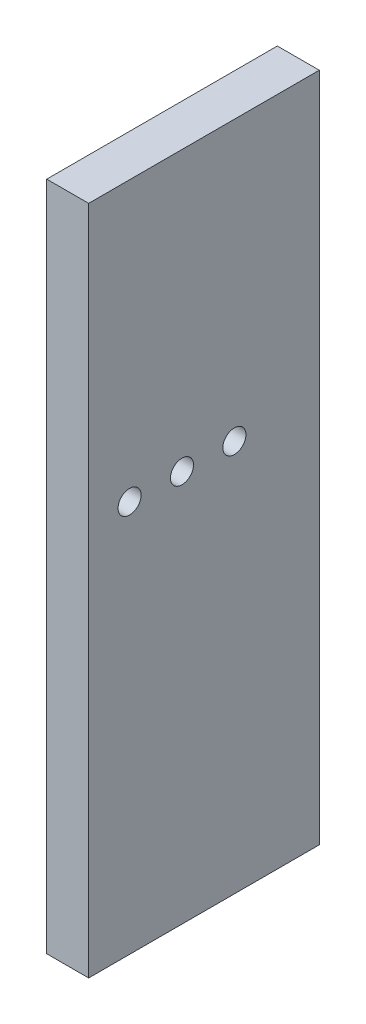
from build123d import *

# Parameters (mm, degrees)
SKETCH1_W                                = 20
SKETCH1_H                                = 320
BOSS_EXTRUDE1_DEPTH                      = 110
CBORE_FOR_M10_HEX_HEAD_BOLT1_D           = 11
CBORE_FOR_M10_HEX_HEAD_BOLT1_DEPTH       = 22.25
CBORE_FOR_M10_HEX_HEAD_BOLT1_CBORE_D     = 15
CBORE_FOR_M10_HEX_HEAD_BOLT1_CBORE_DEPTH = 10
CBORE_FOR_M10_HEX_HEAD_BOLT1_TIP         = 3.304733405


with BuildPart() as part:
    # Sketch1 → Boss-Extrude1 (new body)
    with BuildSketch(Plane.XY):
        with Locations((-110, 300)):
            Rectangle(SKETCH1_W, SKETCH1_H)
    extrude(amount=BOSS_EXTRUDE1_DEPTH)

    # CBORE for M10 Hex Head Bolt1
    with Locations(Plane.ZY.offset(120)):
        with Locations((40.49, 327), (65.49, 327), (90.49, 327)):
            CounterBoreHole(CBORE_FOR_M10_HEX_HEAD_BOLT1_D / 2, CBORE_FOR_M10_HEX_HEAD_BOLT1_CBORE_D / 2, CBORE_FOR_M10_HEX_HEAD_BOLT1_CBORE_DEPTH, depth=CBORE_FOR_M10_HEX_HEAD_BOLT1_DEPTH)
            with Locations((0, 0, -(CBORE_FOR_M10_HEX_HEAD_BOLT1_DEPTH + CBORE_FOR_M10_HEX_HEAD_BOLT1_TIP / 2))):  # 118° drill point
                Cone(0, CBORE_FOR_M10_HEX_HEAD_BOLT1_D / 2, CBORE_FOR_M10_HEX_HEAD_BOLT1_TIP, mode=Mode.SUBTRACT)


solid = part.part
